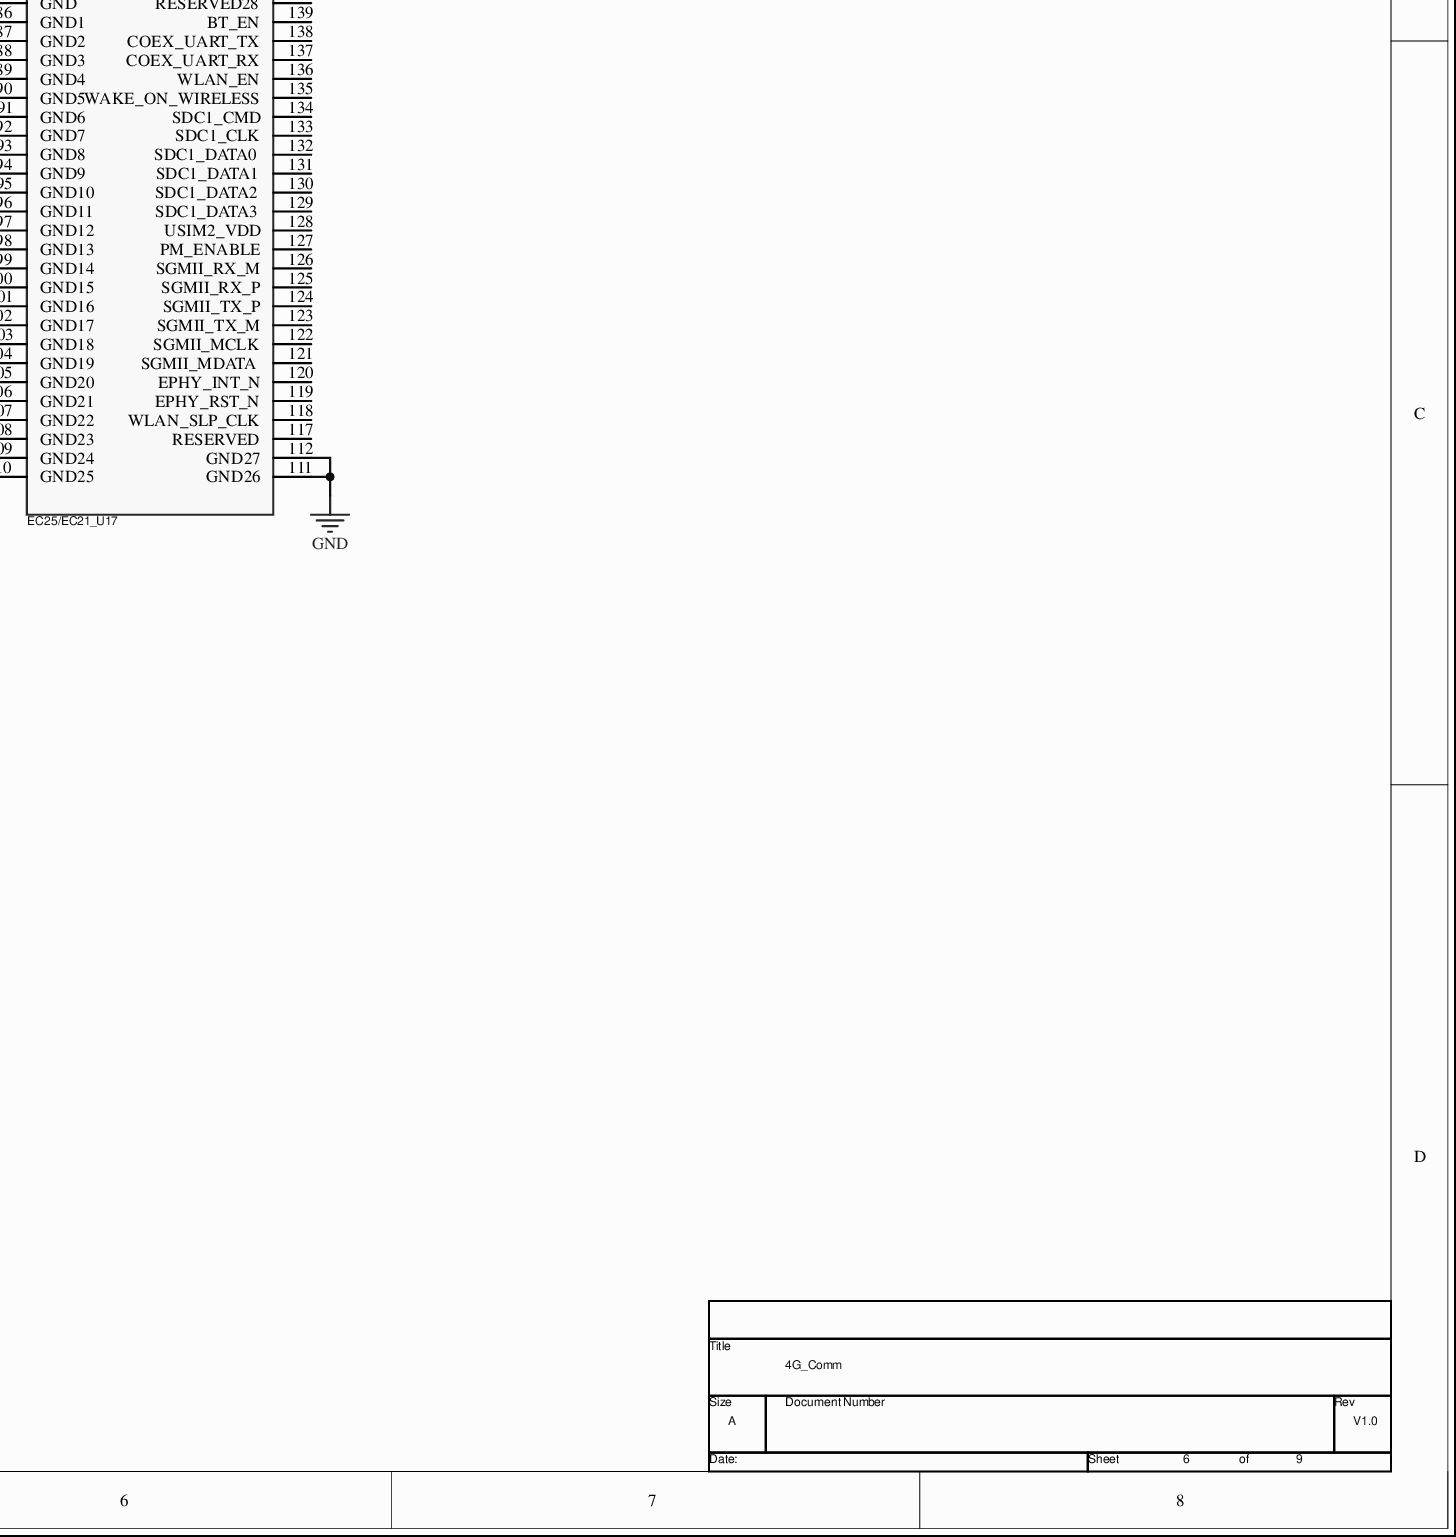
[diagram p0: MISC86294-12.SchDoc, bottom right]
# Altium project MISC86294-22.PrjPcb (part 4 of 5)
## Sheet MISC86294-12.SchDoc (continued)
### Parts (continued)
C81  10nF  [C0603]
C82  33pF/50V  [C0603]
C83  33pF/50V  [C0603]
C84  33pF/50V  [C0603]
C85  33pF/50V  [C0603]
C93  100nF/50V  [C0603]
C122  100nF/50V  [C0603]
C123  33pF/50V  [C0603]
C128  33pF/50V  [C0603]
C129  33pF/50V  [C0603]
C130  33pF/50V  [C0603]
D4  SMAJ6.8CA  [SMA]
D5  SMAJ6.8CA  [SMA]
D6  SMAJ6.8CA  [SMA]
D7  SMAJ6.8CA  [SMA]
D8  GREEN  [LED0805]
D9  GREEN  [LED0805]
D10  GREEN  [LED0805]
J2  MMCX-KE RF connector  [MMCX-KE]
J3  MMCX-KE RF connector  [MMCX-KE]
J4  HEADER 5  [2.54mm_paizhen_5pin]
J23  Boot Option-2.54-single-row pin header  [HDR_1X2_254]
Q3  2SC4617TLQ  [EMT3]
Q4  2SC4617TLQ  [EMT3]
Q5  2SC4617TLQ  [EMT3]
Q6  2SC4617TLQ  [EMT3]
Q7  2SC4617TLQ  [EMT3]
Q8  2SC4617TLQ  [EMT3]
Q9  2SC4617TLQ  [EMT3]
Q10  2SC4617TLQ  [EMT3]
Q11  DTC043ZEBTL  [SOT-416_L1_6-W0_8-P1_00-LS1_6-BR]
Q12  DTC043ZEBTL  [SOT-416_L1_6-W0_8-P1_00-LS1_6-BR]
Q13  DTC043ZEBTL  [SOT-416_L1_6-W0_8-P1_00-LS1_6-BR]
Q14  DTC043ZEBTL  [SOT-416_L1_6-W0_8-P1_00-LS1_6-BR]
Q15  DTC043ZEBTL  [SOT-416_L1_6-W0_8-P1_00-LS1_6-BR]
Q16  DTC043ZEBTL  [SOT-416_L1_6-W0_8-P1_00-LS1_6-BR]
Q17  DTC043ZEBTL  [SOT-416_L1_6-W0_8-P1_00-LS1_6-BR]
R34  4.7K  [R0603]
R35  4.7K  [R0603]
R36  0R  [R0603]
R37  10K  [R0603]
R38  4.7K  [R0603]
R39  10K  [R0603]
R40  10K  [R0603]
R41  0R  [R0603]
R42  10K  [R0603]
R43  0R  [R0603]
R44  10K  [R0603]
R45  4.7K  [R0603]
R46  0R  [R0603]
R47  0R  [R0603]
R48  0R  [R0603]
R49  4.7K  [R0603]
R50  0R  [R0603]
R51  0R  [R0603]
R52  10K  [R0603]
R53  0R  [R0603]
R54  4.7K  [R0603]
R55  10K  [R0603]
R56  4.7K  [R0603]
R57  4.7K  [R0603]
R58  4.7K  [R0603]
R59  47K  [R0603]
R60  100K  [R0603]
R61  330R  [R0603]
R62  NM  [R0603]
R63  47K  [R0603]
R64  4.7K  [R0603]
R65  4.7K  [R0603]
R66  4.7K  [R0603]
R67  22R  [R0603]
R68  22R  [R0603]
R69  22R  [R0603]
R80  22R  [R0603]
R82  22R  [R0603]
R85  10K  [R0603]
R86  10K  [R0603]
R87  10K  [R0603]
R90  22R  [R0603]
R91  NM  [R0603]
U5  EC25/EC21_U17  [EC20]  (parts A,B of 2)
U6  MIC29302WU  [TO-263-5]
U7  China Mobile eSIM  [DFN-8_L6.0-W5.0-P1.27-BL-EP-A]
U8  ESDA6V8V6-6  [SOT-563]
U19  China Telecom eSIM  [DFN-8_L6.0-W5.0-P1.27-BL-EP-A]
U20  FSA2567MPX  [TQFN-16_L3.0-W3.0-P0.50-BL-EP1.7]
U21  ESDA6V8V6-6  [SOT-563]

### Ports
MCU2_CTS3 (in), MCU2_RTS3 (out), MCU2_RXD3 (out), MCU2_TXD3 (in), ON/OFF_MCU (in), RESET_MCU (in), SIM_SEL (in), SLEEP_STATUS (out), UART3_DCD (out), UART3_DTR (in), UART3_RI (out), VBAT_EN (in), W_DISABLE_MCU (in), WAKEUP_IN_MCU (in)

### Nets
GND: C55.1 C56.1 C59.2 C60.2 C61.2 C62.2 C64.2 C65.2 C66.2 C67.2 C69.1 C70.1 C74.2 C75.2 C76.2 C77.2 C78.2 C79.2 C80.2 C81.2 C82.2 C83.2 C84.2 C85.2 C93.2 C122.1 C123.2 C128.2 C129.2 C130.2 D4.1(A) D5.1(A) D6.1(A) D7.1(A) J2.2 J2.3 J2.4 J2.5 J3.2 J3.3 J3.4 J3.5 J4.2 J23.2 Q11.2(E) Q12.2(E) Q13.2(E) Q14.2(E) Q15.2(E) Q16.2(E) Q17.2(E) R61.1 R62.1 R63.1 R85.2 U5.8(GND) U5.9(GND1) U5.19(GND3) U5.22(GND4) U5.36(GND5) U5.46(GND7) U5.48(GND8) U5.50(GND9) U5.51(GND10) U5.52(GND11) U5.53(GND12) U5.54(GND13) U5.56(GND15) U5.72(GND18) U5.85(GND) U5.86(GND1) U5.87(GND2) U5.88(GND3) U5.89(GND4) U5.90(GND5) U5.91(GND6) U5.92(GND7) U5.93(GND8) U5.94(GND9) U5.95(GND10) U5.96(GND11) U5.97(GND12) U5.98(GND13) U5.99(GND14) U5.100(GND15) U5.101(GND16) U5.102(GND17) U5.103(GND18) U5.104(GND19) U5.105(GND20) U5.106(GND21) U5.107(GND22) U5.108(GND23) U5.109(GND24) U5.110(GND25) U5.111(GND26) U5.112(GND27) U6.3(GND) U6.6(GND) U7.1(GND) U7.9(EP) U8.2 U19.1(GND) U19.9(EP) U20.6(GND) U20.17(gnd) U21.2
VDD_3.3: C122.2 R42.2 R44.2 R52.2 R55.2 U20.14(VCC)
VDD_5V: C74.1 C75.1 D9.1(A) D10.1(A) R59.2 U6.2(IN)
VDD_EXT: C54.1 C57.1 C58.1 C63.2 C68.2 C71.2 C72.2 C73.2 R34.2 R35.2 R37.1 R38.2 R39.1 R40.1 R45.1 R49.1 R54.1 R56.1 R57.1 R58.1 U5.7(VDD_EXT)
ANT_DIV: C70.2 R46.1 U5.35(ANT_DIV)
ANT_MAIN: C56.2 R36.1 U5.49(ANT_MAIN)
AP_READY_MODULE: Q10.3(C) R57.2 U5.2(AP_READY)
DBG_RXD: D7.2(K) J4.4 U5.11(DBG_RXD)
DBG_TXD: D6.2(K) J4.5 U5.12(DBG_TXD)
NET_MODE: Q15.1(B) U5.5(NET_MODE)
NET_STATUS: Q16.1(B) U5.6(NET_STATUS)
PWRKEY: C79.1 D5.2(K) J4.3 Q14.3(C) R85.1 U5.21(PWRKEY)
RESET_N: Q13.3(C) U5.20(RESET_N)
STATUS: R64.2 U5.61(STATUS)
USIM_CLK: U5.16(USIM_CLK) U20.8(CLK)
USIM_DATA: U5.15(USIM_DATA) U20.12(DAT)
USIM_GND: U5.10(USIM_GND)
USIM_PRESENCE: R62.2 U5.13(USIM_PRESENCE)
USIM_RST: U5.17(USIM_RST) U20.4(RST)
USIM_VDD: U5.14(USIM_VDD) U20.16(VSIM)
USIMA_CLK: R67.1 U20.9(1CLK)
USIMA_DATA: R69.1 R86.1 U20.13(1DAT)
USIMA_RST: R68.1 U20.5(1RST)
USIMA_VDD: C80.1 C83.1 R86.2 U7.8(VCC) U8.5 U20.1(1VSIM)
USIMB_CLK: R82.1 U20.7(2CLK)
USIMB_DATA: R87.2 R90.1 U20.11(2DAT)
USIMB_RST: R80.1 U20.3(2RST)
USIMB_VDD: C93.1 C128.1 R87.1 U19.8(VCC) U20.15(2VSIM) U21.5
VBAT: C59.1 C60.1 C61.1 C62.1 C64.1 C65.1 C66.1 C67.1 C76.1 C77.1 D4.2(K) D8.1(A) J4.1 R60.2 R61.2 U5.57(VBAT_RF) U5.58(VBAT_RF16) U5.59(VBAT_BB) U5.60(VBAT_BB17) U6.4(OUT)
W_DISABLE_MODULE: C78.1 Q12.3(C) U5.4(W_DISABLE#)
WAKEUP_IN_MODULE: C81.1 Q17.3(C) U5.1(WAKEUP_IN)
NetC54_2: C54.2 Q3.2(B) R34.1
NetC55_2: C55.2 J2.1 R36.2
NetC57_2: C57.2 Q4.2(B) R35.1
NetC58_2: C58.2 Q5.2(B) R38.1
NetC63_1: C63.1 Q6.2(B) R45.2
NetC68_1: C68.1 Q7.2(B) R49.2
NetC69_2: C69.2 J3.1 R46.2
NetC71_1: C71.1 Q8.2(B) R54.2
NetC72_1: C72.1 Q9.2(B) R56.2
NetC73_1: C73.1 Q10.2(B) R58.2
NetC82_1: C82.1 R67.2 U7.6(CLK) U8.3
NetC84_1: C84.1 R68.2 U7.7(RST) U8.1
NetC85_1: C85.1 R69.2 U7.3(I/O) U8.4
NetC123_1: C123.1 R82.2 U19.6(CLK) U21.3
NetC129_1: C129.1 R80.2 U19.7(RST) U21.1
NetC130_1: C130.1 R90.2 U19.3(I/O) U21.4
NetD8_2: D8.2(K) R64.1
NetD9_2: D9.2(K) R65.1
NetD10_2: D10.2(K) R66.1
NetJ17_1: Q4.1(E) ; port MCU2_TXD3
NetJ17_2: Q7.3(C) R44.1 ; port MCU2_RXD3
NetJ23_1: J23.1 R91.1 U20.2(SEL) ; port SIM_SEL
NetQ3_1: Q3.1(E) ; port MCU2_CTS3
NetQ3_3: Q3.3(C) R37.2 R41.1
NetQ4_3: Q4.3(C) R39.2 R53.1
NetQ5_1: Q5.1(E) ; port UART3_DTR
NetQ5_3: Q5.3(C) R40.2 R48.1
NetQ6_1: Q6.1(E) R43.1
NetQ6_3: Q6.3(C) R42.1 ; port MCU2_RTS3
NetQ7_1: Q7.1(E) R51.1
NetQ8_1: Q8.1(E) R47.1
NetQ8_3: Q8.3(C) R52.1 ; port UART3_DCD
NetQ9_1: Q9.1(E) R50.1
NetQ9_3: Q9.3(C) R55.1 ; port UART3_RI
NetQ10_1: Q10.1(E) ; port SLEEP_STATUS
NetQ11_1: Q11.1(B) ; port VBAT_EN
NetQ11_3: Q11.3(C) R59.1 U6.1(EN)
NetQ12_1: Q12.1(B) ; port W_DISABLE_MCU
NetQ13_1: Q13.1(B) ; port RESET_MCU
NetQ14_1: Q14.1(B) ; port ON/OFF_MCU
NetQ15_3: Q15.3(C) R65.2
NetQ16_3: Q16.3(C) R66.2
NetQ17_1: Q17.1(B) ; port WAKEUP_IN_MCU
NetR41_2: R41.2 U5.65(RTS)
NetR43_2: R43.2 U5.64(CTS)
NetR47_2: R47.2 U5.63(DCD)
NetR48_2: R48.2 U5.66(DTR)
NetR50_2: R50.2 U5.62(RI)
NetR51_2: R51.2 U5.67(TXD)
NetR53_2: R53.2 U5.68(RXD)
NetR60_1: R60.1 R63.2 U6.5(ADJ)
NetR91_2: R91.2 U20.10(NC)

Not connected (* = marked no-connect by the designer): U5 3(RVD) 18(RVD2) 23(SD_INS_DET) 24(PCM_IN) 25(PCM_OUT) 26(PCM_SYNC) 27(PCM_CLK) 28(SDC2_DATA3) 29(SDC2_DATA2) 30(SDC2_DATA1) 31(SDC2_DATA0) 32(SDC2_CLK) 33(SDC2_CMD) 34(VDD_SDIO) 37(BT_RTS) 38(BT_TXD) 39(BT_RXD) 40(BT_CTS) 41(I2C_SCL) 42(I2C_SDA) 43(RVD6) 44(ADC1) 45(ADC0) 47(ANT_GNSS) 55(RVD14) 69(USB_DP) 70(USB_DM) 71(USB_VBUS) 113(RVD20) 114(RVD21) 115(USB_BOOT) 116(RVD19) 117(RESERVED) 118(WLAN_SLP_CLK) 119(EPHY_RST_N) 120(EPHY_INT_N) 121(SGMII_MDATA) 122(SGMII_MCLK) 123(SGMII_TX_M) 124(SGMII_TX_P) 125(SGMII_RX_P) 126(SGMII_RX_M) 127(PM_ENABLE) 128(USIM2_VDD) 129(SDC1_DATA3) 130(SDC1_DATA2) 131(SDC1_DATA1) 132(SDC1_DATA0) 133(SDC1_CLK) 134(SDC1_CMD) 135(WAKE_ON_WIRELESS) 136(WLAN_EN) 137(COEX_UART_RX) 138(COEX_UART_TX) 139(BT_EN) 140(RESERVED28) 141(RVD22) 142(RVD23) 143(RVD24) 144(RVD25); U7 2(NC) 4(NC1) 5(NC2); U8 6; U19 2(NC) 4(NC1) 5(NC2); U21 6

### Notes on the sheet
- Main antenna
- Close to VBAT_BB
- Close to VBAT_RF
- (near D4) Diversity receive antenna
- Note: single-ended impedance of RF antenna is 50Ω
- VBAT traces should use a star topology connected to pins VBAT_BB and VBAT_RF
- VBAT supply current must meet 2.0A rated output capability
- VBAT operating voltage range is 3.3V-4.3V
- 4G module LDO
- (near J4) Reserved test point
- VBAT
- Recommended load current not less than 10mA

### Library data of the parts
*#5 = TitleBlock0: Document: Agr-Ctrl-3GS-06; Page Create Date: March  8, 1995
C54 = Cap_C54: Kind: General; SubKind: Capacitor; Origin: Altium; Published: 8-Jun-2000; LatestRevisionDate: 17-Jul-2002; LatestRevisionNote: Re-released for DXP Platform.; PackageReference: RAD-0.3; User_Value: 1nF/50V; Created: 1/08/1993; Spice Prefix: C; Type: Capacitor; Publisher: Altium Limited
C55 = Cap_C97: Kind: General; SubKind: Capacitor; Origin: Altium; Published: 8-Jun-2000; LatestRevisionDate: 17-Jul-2002; LatestRevisionNote: Re-released for DXP Platform.; PackageReference: RAD-0.3; User_Value: NM; Created: 1/08/1993; Spice Prefix: C; Type: Capacitor; Publisher: Altium Limited
C56 = Cap_C98: Kind: General; SubKind: Capacitor; Origin: Altium; Published: 8-Jun-2000; LatestRevisionDate: 17-Jul-2002; LatestRevisionNote: Re-released for DXP Platform.; PackageReference: RAD-0.3; User_Value: NM; Created: 1/08/1993; Spice Prefix: C; Type: Capacitor; Publisher: Altium Limited
C57 = Cap_C109: Kind: General; SubKind: Capacitor; Origin: Altium; Published: 8-Jun-2000; LatestRevisionDate: 17-Jul-2002; LatestRevisionNote: Re-released for DXP Platform.; PackageReference: RAD-0.3; User_Value: 1nF/50V; Created: 1/08/1993; Spice Prefix: C; Type: Capacitor; Publisher: Altium Limited
C58 = Cap_C113: Kind: General; SubKind: Capacitor; Origin: Altium; Published: 8-Jun-2000; LatestRevisionDate: 17-Jul-2002; LatestRevisionNote: Re-released for DXP Platform.; PackageReference: RAD-0.3; User_Value: 1nF/50V; Created: 1/08/1993; Spice Prefix: C; Type: Capacitor; Publisher: Altium Limited
C59 = Cap2_C77: Origin: Altium; Published: 23-Sep-2002; PackageReference: CAPR5-4X5; User_Value: 100uF/10V; Publisher: Altium Limited
C60 = Cap_C73: Kind: General; SubKind: Capacitor; Origin: Altium; Published: 8-Jun-2000; LatestRevisionDate: 17-Jul-2002; LatestRevisionNote: Re-released for DXP Platform.; PackageReference: RAD-0.3; User_Value: 100nF/50V; Created: 1/08/1993; Spice Prefix: C; Type: Capacitor; Publisher: Altium Limited
C61 = Cap_C74: Kind: General; SubKind: Capacitor; Origin: Altium; Published: 8-Jun-2000; LatestRevisionDate: 17-Jul-2002; LatestRevisionNote: Re-released for DXP Platform.; PackageReference: RAD-0.3; User_Value: 33pF/50V; Created: 1/08/1993; Spice Prefix: C; Type: Capacitor; Publisher: Altium Limited
C62 = Cap_C75: Kind: General; SubKind: Capacitor; Origin: Altium; Published: 8-Jun-2000; LatestRevisionDate: 17-Jul-2002; LatestRevisionNote: Re-released for DXP Platform.; PackageReference: RAD-0.3; User_Value: 12pF/50V; Created: 1/08/1993; Spice Prefix: C; Type: Capacitor; Publisher: Altium Limited
C63 = Cap_C114: Kind: General; SubKind: Capacitor; Origin: Altium; Published: 8-Jun-2000; LatestRevisionDate: 17-Jul-2002; LatestRevisionNote: Re-released for DXP Platform.; PackageReference: RAD-0.3; User_Value: 1nF/50V; Created: 1/08/1993; Spice Prefix: C; Type: Capacitor; Publisher: Altium Limited
C64 = Cap2_C76: Origin: Altium; Published: 23-Sep-2002; PackageReference: CAPR5-4X5; User_Value: 100uF/10V; Publisher: Altium Limited
C65 = Cap_C70: Kind: General; SubKind: Capacitor; Origin: Altium; Published: 8-Jun-2000; LatestRevisionDate: 17-Jul-2002; LatestRevisionNote: Re-released for DXP Platform.; PackageReference: RAD-0.3; User_Value: 100nF/50V; Created: 1/08/1993; Spice Prefix: C; Type: Capacitor; Publisher: Altium Limited
C66 = Cap_C71: Kind: General; SubKind: Capacitor; Origin: Altium; Published: 8-Jun-2000; LatestRevisionDate: 17-Jul-2002; LatestRevisionNote: Re-released for DXP Platform.; PackageReference: RAD-0.3; User_Value: 33pF/50V; Created: 1/08/1993; Spice Prefix: C; Type: Capacitor; Publisher: Altium Limited
C67 = Cap_C72: Kind: General; SubKind: Capacitor; Origin: Altium; Published: 8-Jun-2000; LatestRevisionDate: 17-Jul-2002; LatestRevisionNote: Re-released for DXP Platform.; PackageReference: RAD-0.3; User_Value: 12pF/50V; Created: 1/08/1993; Spice Prefix: C; Type: Capacitor; Publisher: Altium Limited
C68 = Cap_C115: Kind: General; SubKind: Capacitor; Origin: Altium; Published: 8-Jun-2000; LatestRevisionDate: 17-Jul-2002; LatestRevisionNote: Re-released for DXP Platform.; PackageReference: RAD-0.3; User_Value: 1nF/50V; Created: 1/08/1993; Spice Prefix: C; Type: Capacitor; Publisher: Altium Limited
C69 = Cap_C102: Kind: General; SubKind: Capacitor; Origin: Altium; Published: 8-Jun-2000; LatestRevisionDate: 17-Jul-2002; LatestRevisionNote: Re-released for DXP Platform.; PackageReference: RAD-0.3; User_Value: NM; Created: 1/08/1993; Spice Prefix: C; Type: Capacitor; Publisher: Altium Limited
C70 = Cap_C103: Kind: General; SubKind: Capacitor; Origin: Altium; Published: 8-Jun-2000; LatestRevisionDate: 17-Jul-2002; LatestRevisionNote: Re-released for DXP Platform.; PackageReference: RAD-0.3; User_Value: NM; Created: 1/08/1993; Spice Prefix: C; Type: Capacitor; Publisher: Altium Limited
C71 = Cap_C116: Kind: General; SubKind: Capacitor; Origin: Altium; Published: 8-Jun-2000; LatestRevisionDate: 17-Jul-2002; LatestRevisionNote: Re-released for DXP Platform.; PackageReference: RAD-0.3; User_Value: 1nF/50V; Created: 1/08/1993; Spice Prefix: C; Type: Capacitor; Publisher: Altium Limited
C72 = Cap_C117: Kind: General; SubKind: Capacitor; Origin: Altium; Published: 8-Jun-2000; LatestRevisionDate: 17-Jul-2002; LatestRevisionNote: Re-released for DXP Platform.; PackageReference: RAD-0.3; User_Value: 1nF/50V; Created: 1/08/1993; Spice Prefix: C; Type: Capacitor; Publisher: Altium Limited
C73 = Cap_C58: Kind: General; SubKind: Capacitor; Origin: Altium; Published: 8-Jun-2000; LatestRevisionDate: 17-Jul-2002; LatestRevisionNote: Re-released for DXP Platform.; PackageReference: RAD-0.3; User_Value: 1nF/50V; Created: 1/08/1993; Spice Prefix: C; Type: Capacitor; Publisher: Altium Limited
C74 = Cap_C91: Origin: Altium; Published: 8-Jun-2000; LatestRevisionDate: 17-Jul-2002; LatestRevisionNote: Re-released for DXP Platform.; PackageReference: RAD-0.3; User_Value: 470uF/25V; Created: 1/08/1993; Publisher: Altium Limited
C75 = Cap_C101: Kind: General; SubKind: Capacitor; Origin: Altium; Published: 8-Jun-2000; LatestRevisionDate: 17-Jul-2002; LatestRevisionNote: Re-released for DXP Platform.; PackageReference: RAD-0.3; User_Value: 100nF/50V; Created: 1/08/1993; Spice Prefix: C; Type: Capacitor; Publisher: Altium Limited
C76 = Cap_C104: Origin: Altium; Published: 8-Jun-2000; LatestRevisionDate: 17-Jul-2002; LatestRevisionNote: Re-released for DXP Platform.; PackageReference: RAD-0.3; User_Value: 470uF/25V; Created: 1/08/1993; Publisher: Altium Limited
C77 = Cap_C105: Kind: General; SubKind: Capacitor; Origin: Altium; Published: 8-Jun-2000; LatestRevisionDate: 17-Jul-2002; LatestRevisionNote: Re-released for DXP Platform.; PackageReference: RAD-0.3; User_Value: 100nF/50V; Created: 1/08/1993; Spice Prefix: C; Type: Capacitor; Publisher: Altium Limited
C78 = Cap_C48_Dup1: Kind: General; SubKind: Capacitor; Origin: Altium; Published: 8-Jun-2000; LatestRevisionDate: 17-Jul-2002; LatestRevisionNote: Re-released for DXP Platform.; PackageReference: RAD-0.3; User_Value: 10nF; Created: 1/08/1993; Spice Prefix: C; Type: Capacitor; Publisher: Altium Limited
C79 = Cap_C32_Dup1: Kind: General; SubKind: Capacitor; Origin: Altium; Published: 8-Jun-2000; LatestRevisionDate: 17-Jul-2002; LatestRevisionNote: Re-released for DXP Platform.; PackageReference: RAD-0.3; User_Value: 10nF; Created: 1/08/1993; Spice Prefix: C; Type: Capacitor; Publisher: Altium Limited
C80 C93 = Cap_C45_Dup1: Kind: General; SubKind: Capacitor; Origin: Altium; Published: 8-Jun-2000; LatestRevisionDate: 17-Jul-2002; LatestRevisionNote: Re-released for DXP Platform.; PackageReference: RAD-0.3; User_Value: 100nF/50V; Created: 1/08/1993; Spice Prefix: C; Type: Capacitor; Publisher: Altium Limited
C81 = Cap_C47_Dup1: Kind: General; SubKind: Capacitor; Origin: Altium; Published: 8-Jun-2000; LatestRevisionDate: 17-Jul-2002; LatestRevisionNote: Re-released for DXP Platform.; PackageReference: RAD-0.3; User_Value: 10nF; Created: 1/08/1993; Spice Prefix: C; Type: Capacitor; Publisher: Altium Limited
C82 C123 = Cap_C51_Dup1: Kind: General; SubKind: Capacitor; Origin: Altium; Published: 8-Jun-2000; LatestRevisionDate: 17-Jul-2002; LatestRevisionNote: Re-released for DXP Platform.; PackageReference: RAD-0.3; User_Value: 33pF/50V; Created: 1/08/1993; Spice Prefix: C; Type: Capacitor; Publisher: Altium Limited
C83 C128 = Cap_C49_Dup1: Kind: General; SubKind: Capacitor; Origin: Altium; Published: 8-Jun-2000; LatestRevisionDate: 17-Jul-2002; LatestRevisionNote: Re-released for DXP Platform.; PackageReference: RAD-0.3; User_Value: 33pF/50V; Created: 1/08/1993; Spice Prefix: C; Type: Capacitor; Publisher: Altium Limited
C84 C129 = Cap_C50: Kind: General; SubKind: Capacitor; Origin: Altium; Published: 8-Jun-2000; LatestRevisionDate: 17-Jul-2002; LatestRevisionNote: Re-released for DXP Platform.; PackageReference: RAD-0.3; User_Value: 33pF/50V; Created: 1/08/1993; Spice Prefix: C; Type: Capacitor; Publisher: Altium Limited
C85 C130 = Cap_C52_Dup1: Kind: General; SubKind: Capacitor; Origin: Altium; Published: 8-Jun-2000; LatestRevisionDate: 17-Jul-2002; LatestRevisionNote: Re-released for DXP Platform.; PackageReference: RAD-0.3; User_Value: 33pF/50V; Created: 1/08/1993; Spice Prefix: C; Type: Capacitor; Publisher: Altium Limited
C122 = Cap: SMD ceramic capacitor; Published: 8-Jun-2000; LatestRevisionDate: 17-Jul-2002; LatestRevisionNote: Re-released for DXP Platform.; PackageReference: RAD-0.3; Value: 100nF/50V; Publisher: Altium Limited
D4 = Diode_1_D8: Origin: Altium; Published: 8-Jun-2000; LatestRevisionDate: 17-Jul-2002; LatestRevisionNote: Re-released for DXP Platform.; PackageVersion: Sep-1996; PackageReference: SMC; Code_JEDEC: DO-214-AB; Publisher: Altium Limited
D5 = Diode_1_D14: Origin: Altium; Published: 8-Jun-2000; LatestRevisionDate: 17-Jul-2002; LatestRevisionNote: Re-released for DXP Platform.; PackageVersion: Sep-1996; PackageReference: SMC; Code_JEDEC: DO-214-AB; Publisher: Altium Limited
D6 = Diode_1_D15: Origin: Altium; Published: 8-Jun-2000; LatestRevisionDate: 17-Jul-2002; LatestRevisionNote: Re-released for DXP Platform.; PackageVersion: Sep-1996; PackageReference: SMC; Code_JEDEC: DO-214-AB; Publisher: Altium Limited
D7 = Diode_1_D16: Origin: Altium; Published: 8-Jun-2000; LatestRevisionDate: 17-Jul-2002; LatestRevisionNote: Re-released for DXP Platform.; PackageVersion: Sep-1996; PackageReference: SMC; Code_JEDEC: DO-214-AB; Publisher: Altium Limited
D8 = LED1_D21: Origin: Altium; Published: 8-Jun-2000; LatestRevisionDate: 08-Jul-2005; LatestRevisionNote: Mech Layer 1 removed.; PackageReference: LED-1; Publisher: Altium Limited
D9 = LED1_D22: Origin: Altium; Published: 8-Jun-2000; LatestRevisionDate: 08-Jul-2005; LatestRevisionNote: Mech Layer 1 removed.; PackageReference: LED-1; Publisher: Altium Limited
D10 = LED1_D23: Origin: Altium; Published: 8-Jun-2000; LatestRevisionDate: 08-Jul-2005; LatestRevisionNote: Mech Layer 1 removed.; PackageReference: LED-1; Publisher: Altium Limited
J2 = CIRCLE_J19: Origin: Altium
J3 = CIRCLE_J21: Origin: Altium
J23 = HEADER 2
Q3-Q10 = 2SC4617TLQ: PspiceTemplate: Q^@REFDES %C %B %E
Q11 = DTC043ZEBTL_Q10: BOM_Manufacturer: ROHM; BOM_Paste Type: expand; Origin: Altium; BOM_Supplier: LCSC; BOM_Manufacturer Part: DTC043ZEBTL; BOM_Supplier Part: C96459; spicePre: Q; spiceSymbolName: DTC043ZEBTL
Q12 = DTC043ZEBTL_Q6: BOM_Manufacturer: ROHM; BOM_Paste Type: expand; Origin: Altium; BOM_Supplier: LCSC; BOM_Manufacturer Part: DTC043ZEBTL; BOM_Supplier Part: C96459; spicePre: Q; spiceSymbolName: DTC043ZEBTL
Q13 = DTC043ZEBTL_Q4: BOM_Manufacturer: ROHM; BOM_Paste Type: expand; Origin: Altium; BOM_Supplier: LCSC; BOM_Manufacturer Part: DTC043ZEBTL; BOM_Supplier Part: C96459; spicePre: Q; spiceSymbolName: DTC043ZEBTL
Q14 = DTC043ZEBTL_Q3: BOM_Manufacturer: ROHM; BOM_Paste Type: expand; Origin: Altium; BOM_Supplier: LCSC; BOM_Manufacturer Part: DTC043ZEBTL; BOM_Supplier Part: C96459; spicePre: Q; spiceSymbolName: DTC043ZEBTL
Q15 = DTC043ZEBTL_Q12: BOM_Manufacturer: ROHM; BOM_Paste Type: expand; Origin: Altium; BOM_Supplier: LCSC; BOM_Manufacturer Part: DTC043ZEBTL; BOM_Supplier Part: C96459; spicePre: Q; spiceSymbolName: DTC043ZEBTL
Q16 = DTC043ZEBTL_Q13: BOM_Manufacturer: ROHM; BOM_Paste Type: expand; Origin: Altium; BOM_Supplier: LCSC; BOM_Manufacturer Part: DTC043ZEBTL; BOM_Supplier Part: C96459; spicePre: Q; spiceSymbolName: DTC043ZEBTL
Q17 = DTC043ZEBTL_Q5: BOM_Manufacturer: ROHM; BOM_Paste Type: expand; Origin: Altium; BOM_Supplier: LCSC; BOM_Manufacturer Part: DTC043ZEBTL; BOM_Supplier Part: C96459; spicePre: Q; spiceSymbolName: DTC043ZEBTL
R34 = Res1_R99: Kind: General; SubKind: Resistor; Origin: Altium; Published: 8-Jun-2000; LatestRevisionDate: 17-Jul-2002; LatestRevisionNote: Re-released for DXP Platform.; PackageReference: AXIAL-0.3; User_Value: 4.7K; Created: 1/08/1993; Spice Prefix: R; Type: Resistor; Publisher: Altium Limited
R35 = Res1_R100: Kind: General; SubKind: Resistor; Origin: Altium; Published: 8-Jun-2000; LatestRevisionDate: 17-Jul-2002; LatestRevisionNote: Re-released for DXP Platform.; PackageReference: AXIAL-0.3; User_Value: 4.7K; Created: 1/08/1993; Spice Prefix: R; Type: Resistor; Publisher: Altium Limited
R36 = Res1_R62: Kind: General; SubKind: Resistor; Origin: Altium; Published: 8-Jun-2000; LatestRevisionDate: 17-Jul-2002; LatestRevisionNote: Re-released for DXP Platform.; PackageReference: AXIAL-0.3; User_Value: 0R; Created: 1/08/1993; Spice Prefix: R; Type: Resistor; Publisher: Altium Limited
R37 = Res1_R101: Kind: General; SubKind: Resistor; Origin: Altium; Published: 8-Jun-2000; LatestRevisionDate: 17-Jul-2002; LatestRevisionNote: Re-released for DXP Platform.; PackageReference: AXIAL-0.3; User_Value: 10K; Created: 1/08/1993; Spice Prefix: R; Type: Resistor; Publisher: Altium Limited
R38 = Res1_R102: Kind: General; SubKind: Resistor; Origin: Altium; Published: 8-Jun-2000; LatestRevisionDate: 17-Jul-2002; LatestRevisionNote: Re-released for DXP Platform.; PackageReference: AXIAL-0.3; User_Value: 4.7K; Created: 1/08/1993; Spice Prefix: R; Type: Resistor; Publisher: Altium Limited
R39 = Res1_R103: Kind: General; SubKind: Resistor; Origin: Altium; Published: 8-Jun-2000; LatestRevisionDate: 17-Jul-2002; LatestRevisionNote: Re-released for DXP Platform.; PackageReference: AXIAL-0.3; User_Value: 10K; Created: 1/08/1993; Spice Prefix: R; Type: Resistor; Publisher: Altium Limited
R40 = Res1_R104: Kind: General; SubKind: Resistor; Origin: Altium; Published: 8-Jun-2000; LatestRevisionDate: 17-Jul-2002; LatestRevisionNote: Re-released for DXP Platform.; PackageReference: AXIAL-0.3; User_Value: 10K; Created: 1/08/1993; Spice Prefix: R; Type: Resistor; Publisher: Altium Limited
R41 = Res1_R26_Dup1: Kind: General; SubKind: Resistor; Origin: Altium; Published: 8-Jun-2000; LatestRevisionDate: 17-Jul-2002; LatestRevisionNote: Re-released for DXP Platform.; PackageReference: AXIAL-0.3; User_Value: 0R; Created: 1/08/1993; Spice Prefix: R; Type: Resistor; Publisher: Altium Limited
R42 = Res1_R105: Kind: General; SubKind: Resistor; Origin: Altium; Published: 8-Jun-2000; LatestRevisionDate: 17-Jul-2002; LatestRevisionNote: Re-released for DXP Platform.; PackageReference: AXIAL-0.3; User_Value: 10K; Created: 1/08/1993; Spice Prefix: R; Type: Resistor; Publisher: Altium Limited
R43 = Res1_R106: Kind: General; SubKind: Resistor; Origin: Altium; Published: 8-Jun-2000; LatestRevisionDate: 17-Jul-2002; LatestRevisionNote: Re-released for DXP Platform.; PackageReference: AXIAL-0.3; User_Value: 0R; Created: 1/08/1993; Spice Prefix: R; Type: Resistor; Publisher: Altium Limited
R44 = Res1_R108: Kind: General; SubKind: Resistor; Origin: Altium; Published: 8-Jun-2000; LatestRevisionDate: 17-Jul-2002; LatestRevisionNote: Re-released for DXP Platform.; PackageReference: AXIAL-0.3; User_Value: 10K; Created: 1/08/1993; Spice Prefix: R; Type: Resistor; Publisher: Altium Limited
R45 = Res1_R107: Kind: General; SubKind: Resistor; Origin: Altium; Published: 8-Jun-2000; LatestRevisionDate: 17-Jul-2002; LatestRevisionNote: Re-released for DXP Platform.; PackageReference: AXIAL-0.3; User_Value: 4.7K; Created: 1/08/1993; Spice Prefix: R; Type: Resistor; Publisher: Altium Limited
R46 = Res1_R64: Kind: General; SubKind: Resistor; Origin: Altium; Published: 8-Jun-2000; LatestRevisionDate: 17-Jul-2002; LatestRevisionNote: Re-released for DXP Platform.; PackageReference: AXIAL-0.3; User_Value: 0R; Created: 1/08/1993; Spice Prefix: R; Type: Resistor; Publisher: Altium Limited
R47 = Res1_R109: Kind: General; SubKind: Resistor; Origin: Altium; Published: 8-Jun-2000; LatestRevisionDate: 17-Jul-2002; LatestRevisionNote: Re-released for DXP Platform.; PackageReference: AXIAL-0.3; User_Value: 0R; Created: 1/08/1993; Spice Prefix: R; Type: Resistor; Publisher: Altium Limited
R48 = Res1_R27_Dup1: Kind: General; SubKind: Resistor; Origin: Altium; Published: 8-Jun-2000; LatestRevisionDate: 17-Jul-2002; LatestRevisionNote: Re-released for DXP Platform.; PackageReference: AXIAL-0.3; User_Value: 0R; Created: 1/08/1993; Spice Prefix: R; Type: Resistor; Publisher: Altium Limited
R49 = Res1_R110: Kind: General; SubKind: Resistor; Origin: Altium; Published: 8-Jun-2000; LatestRevisionDate: 17-Jul-2002; LatestRevisionNote: Re-released for DXP Platform.; PackageReference: AXIAL-0.3; User_Value: 4.7K; Created: 1/08/1993; Spice Prefix: R; Type: Resistor; Publisher: Altium Limited
R50 = Res1_R111: Kind: General; SubKind: Resistor; Origin: Altium; Published: 8-Jun-2000; LatestRevisionDate: 17-Jul-2002; LatestRevisionNote: Re-released for DXP Platform.; PackageReference: AXIAL-0.3; User_Value: 0R; Created: 1/08/1993; Spice Prefix: R; Type: Resistor; Publisher: Altium Limited
R51 = Res1_R28_Dup1: Kind: General; SubKind: Resistor; Origin: Altium; Published: 8-Jun-2000; LatestRevisionDate: 17-Jul-2002; LatestRevisionNote: Re-released for DXP Platform.; PackageReference: AXIAL-0.3; User_Value: 0R; Created: 1/08/1993; Spice Prefix: R; Type: Resistor; Publisher: Altium Limited
R52 = Res1_R112: Kind: General; SubKind: Resistor; Origin: Altium; Published: 8-Jun-2000; LatestRevisionDate: 17-Jul-2002; LatestRevisionNote: Re-released for DXP Platform.; PackageReference: AXIAL-0.3; User_Value: 10K; Created: 1/08/1993; Spice Prefix: R; Type: Resistor; Publisher: Altium Limited
R53 = Res1_R32: Kind: General; SubKind: Resistor; Origin: Altium; Published: 8-Jun-2000; LatestRevisionDate: 17-Jul-2002; LatestRevisionNote: Re-released for DXP Platform.; PackageReference: AXIAL-0.3; User_Value: 0R; Created: 1/08/1993; Spice Prefix: R; Type: Resistor; Publisher: Altium Limited
R54 = Res1_R113: Kind: General; SubKind: Resistor; Origin: Altium; Published: 8-Jun-2000; LatestRevisionDate: 17-Jul-2002; LatestRevisionNote: Re-released for DXP Platform.; PackageReference: AXIAL-0.3; User_Value: 4.7K; Created: 1/08/1993; Spice Prefix: R; Type: Resistor; Publisher: Altium Limited
R55 R85 = Res1_R114: Kind: General; SubKind: Resistor; Origin: Altium; Published: 8-Jun-2000; LatestRevisionDate: 17-Jul-2002; LatestRevisionNote: Re-released for DXP Platform.; PackageReference: AXIAL-0.3; User_Value: 10K; Created: 1/08/1993; Spice Prefix: R; Type: Resistor; Publisher: Altium Limited
R56 = Res1_R115: Kind: General; SubKind: Resistor; Origin: Altium; Published: 8-Jun-2000; LatestRevisionDate: 17-Jul-2002; LatestRevisionNote: Re-released for DXP Platform.; PackageReference: AXIAL-0.3; User_Value: 4.7K; Created: 1/08/1993; Spice Prefix: R; Type: Resistor; Publisher: Altium Limited
R57 = Res1_R30: Kind: General; SubKind: Resistor; Origin: Altium; Published: 8-Jun-2000; LatestRevisionDate: 17-Jul-2002; LatestRevisionNote: Re-released for DXP Platform.; PackageReference: AXIAL-0.3; User_Value: 4.7K; Created: 1/08/1993; Spice Prefix: R; Type: Resistor; Publisher: Altium Limited
R58 = Res1_R31: Kind: General; SubKind: Resistor; Origin: Altium; Published: 8-Jun-2000; LatestRevisionDate: 17-Jul-2002; LatestRevisionNote: Re-released for DXP Platform.; PackageReference: AXIAL-0.3; User_Value: 4.7K; Created: 1/08/1993; Spice Prefix: R; Type: Resistor; Publisher: Altium Limited
R59 = Res1_R65: Kind: General; SubKind: Resistor; Origin: Altium; Published: 8-Jun-2000; LatestRevisionDate: 17-Jul-2002; LatestRevisionNote: Re-released for DXP Platform.; PackageReference: AXIAL-0.3; User_Value: 47K; Created: 1/08/1993; Spice Prefix: R; Type: Resistor; Publisher: Altium Limited
R60 = Res1_R66: Kind: General; SubKind: Resistor; Origin: Altium; Published: 8-Jun-2000; LatestRevisionDate: 17-Jul-2002; LatestRevisionNote: Re-released for DXP Platform.; PackageReference: AXIAL-0.3; User_Value: 100K; Created: 1/08/1993; Spice Prefix: R; Type: Resistor; Publisher: Altium Limited
R61 = Res1_R67: Kind: General; SubKind: Resistor; Origin: Altium; Published: 8-Jun-2000; LatestRevisionDate: 17-Jul-2002; LatestRevisionNote: Re-released for DXP Platform.; PackageReference: AXIAL-0.3; User_Value: 330R; Created: 1/08/1993; Spice Prefix: R; Type: Resistor; Publisher: Altium Limited
R62 = Res1_R42: Kind: General; SubKind: Resistor; Origin: Altium; Published: 8-Jun-2000; LatestRevisionDate: 17-Jul-2002; LatestRevisionNote: Re-released for DXP Platform.; PackageReference: AXIAL-0.3; User_Value: NM; Created: 1/08/1993; Spice Prefix: R; Type: Resistor; Publisher: Altium Limited
R63 = Res1_R68: Kind: General; SubKind: Resistor; Origin: Altium; Published: 8-Jun-2000; LatestRevisionDate: 17-Jul-2002; LatestRevisionNote: Re-released for DXP Platform.; PackageReference: AXIAL-0.3; User_Value: 47K; Created: 1/08/1993; Spice Prefix: R; Type: Resistor; Publisher: Altium Limited
R64 = Res1_R78: Kind: General; SubKind: Resistor; Origin: Altium; Published: 8-Jun-2000; LatestRevisionDate: 17-Jul-2002; LatestRevisionNote: Re-released for DXP Platform.; PackageReference: AXIAL-0.3; User_Value: 4.7K; Created: 1/08/1993; Spice Prefix: R; Type: Resistor; Publisher: Altium Limited
R65 = Res1_R79: Kind: General; SubKind: Resistor; Origin: Altium; Published: 8-Jun-2000; LatestRevisionDate: 17-Jul-2002; LatestRevisionNote: Re-released for DXP Platform.; PackageReference: AXIAL-0.3; User_Value: 4.7K; Created: 1/08/1993; Spice Prefix: R; Type: Resistor; Publisher: Altium Limited
R66 = Res1_R80: Kind: General; SubKind: Resistor; Origin: Altium; Published: 8-Jun-2000; LatestRevisionDate: 17-Jul-2002; LatestRevisionNote: Re-released for DXP Platform.; PackageReference: AXIAL-0.3; User_Value: 4.7K; Created: 1/08/1993; Spice Prefix: R; Type: Resistor; Publisher: Altium Limited
R67 R82 = Res1_R23: Kind: General; SubKind: Resistor; Origin: Altium; Published: 8-Jun-2000; LatestRevisionDate: 17-Jul-2002; LatestRevisionNote: Re-released for DXP Platform.; PackageReference: AXIAL-0.3; User_Value: 22R; Created: 1/08/1993; Spice Prefix: R; Type: Resistor; Publisher: Altium Limited
R68 R80 R86 R87 = Res1_R21_Dup1: Kind: General; SubKind: Resistor; Origin: Altium; Published: 8-Jun-2000; LatestRevisionDate: 17-Jul-2002; LatestRevisionNote: Re-released for DXP Platform.; PackageReference: AXIAL-0.3; Created: 1/08/1993; Spice Prefix: R; Type: Resistor; Publisher: Altium Limited
  R68 R80: User_Value: 22R
  R86 R87: User_Value: 10K
R69 R90 = Res1_R24: Kind: General; SubKind: Resistor; Origin: Altium; Published: 8-Jun-2000; LatestRevisionDate: 17-Jul-2002; LatestRevisionNote: Re-released for DXP Platform.; PackageReference: AXIAL-0.3; User_Value: 22R; Created: 1/08/1993; Spice Prefix: R; Type: Resistor; Publisher: Altium Limited
R91 = Res1: Resistor; Published: 8-Jun-2000; LatestRevisionDate: 17-Jul-2002; LatestRevisionNote: Re-released for DXP Platform.; PackageReference: AXIAL-0.3; Value: NM; Publisher: Altium Limited
U5 = EC25/EC21_U17: Origin: Altium
U6 = MIC29302WU_U22: Origin: Altium
U7 U19 = SIM-A_U25: Origin: Altium
U8 U21 = ESDA6V8V6-6_U26: Origin: Altium
U20 = FSA2567